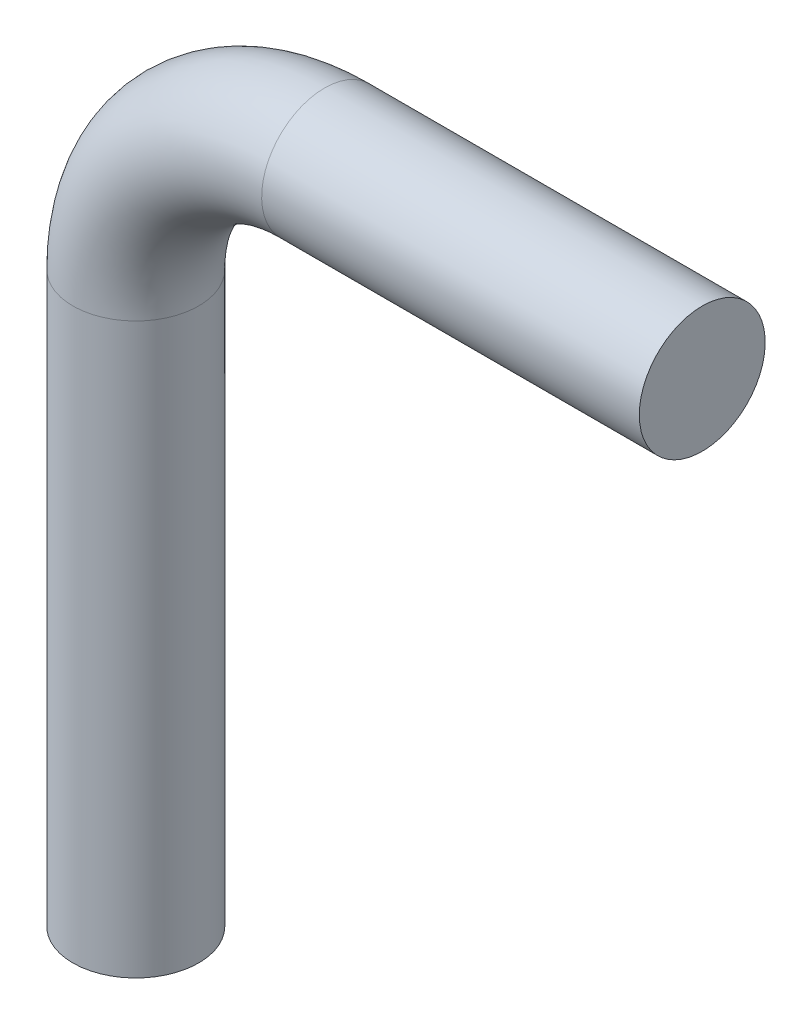
SolidWorks part; units mm, degrees
material "普通碳钢"
ref_plane "Front Plane" through (0, 0, 0) normal (0, 0, 1) x (1, 0, 0)
ref_plane "Top Plane" through (0, 0, 0) normal (0, 1, 0) x (1, 0, 0)
ref_plane "Right Plane" through (0, 0, 0) normal (1, 0, 0) x (0, 0, -1)
sketch "Sketch1" plane through (0, 0, 0) normal (0, 0, 1) x (1, 0, 0)
  line L0 (0, 0) -> (0, 28.702)
  line L1 (0, -55) -> (0, 55) construction
  line L2 (9.525, 38.227) -> (28.575, 38.227)
  line L3 (55, 0) -> (-55, 0) construction
  arc A0 (0, 28.702) -> (9.525, 38.227) centre (9.525, 28.702) cw
  point P10 (0, 38.227)
  dimension "D3" = 9.525
  dimension "D1" = 38.227
  dimension "D2" = 28.575
sketch "Sketch2" plane through (0, 0, 0) normal (0, 1, 0) x (1, 0, 0)
  circle A0 centre (0, 0) radius 3.175
  dimension "D1" = 6.35
sweep "Sweep1" add profiles "Sketch2" path "Sketch1"
